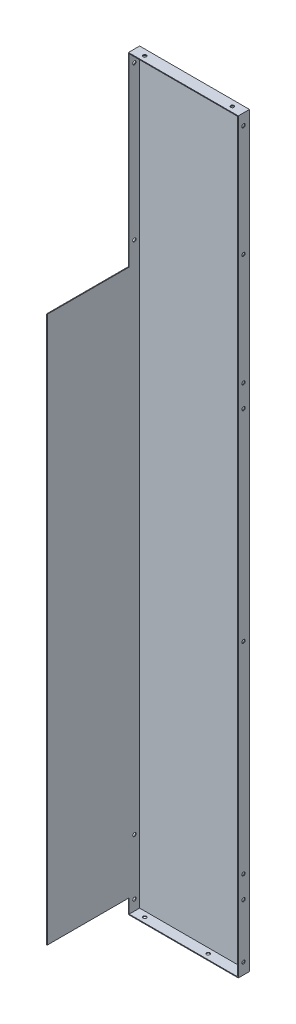
from build123d import *

# Parameters (mm, degrees)
SKETCH_1_W          = 295
SKETCH_1_H          = 2005
EXTRUDE_1_DEPTH     = 30
SHELL_1_T           = -2
SKETCH_2_W          = 2
SKETCH_2_H          = 1467
EXTRUDE_2_DEPTH     = 220
SKETCH_3_R          = 4.5
CUT_EXTRUDE_1_DEPTH = 10
SKETCH_4_R          = 4.5
CUT_EXTRUDE_2_DEPTH = 116
SKETCH_5_R          = 4.5
CUT_EXTRUDE_3_DEPTH = 72
SKETCH_6_R          = 4.5
CUT_EXTRUDE_4_DEPTH = 10
CUT_EXTRUDE_START   = -10
SKETCH_7_R          = 4.5
CUT_EXTRUDE_5_DEPTH = 10
SKETCH_8_R          = 4.5
CUT_EXTRUDE_6_DEPTH = 16


with BuildPart() as part:
    # 草图1 → 凸台-拉伸1 (new body)
    with BuildSketch(Plane.XY):
        with Locations((147.5, 1002.5)):
            Rectangle(SKETCH_1_W, SKETCH_1_H)
    extrude(amount=EXTRUDE_1_DEPTH)

    # 抽壳1
    shell_1_openings = [part.faces().sort_by_distance(p)[0] for p in [
        (147.5, 1002.5, 30),
    ]]
    offset(amount=SHELL_1_T, openings=shell_1_openings, kind=Kind.INTERSECTION)

    # 草图2 → 凸台-拉伸2 (add)
    with BuildSketch(Plane.XY.offset(30)):
        with Locations((1, 773.5)):
            Rectangle(SKETCH_2_W, SKETCH_2_H)
    extrude(amount=EXTRUDE_2_DEPTH)

    # 草图3 → 切除-拉伸1 (cut)
    with BuildSketch(Plane(origin=(0, 2, 0), x_dir=(1, 0, 0), z_dir=(0, 1, 0))):
        with Locations(Location((30, -16, 0), (0, 0, 270))):
            Circle(SKETCH_3_R)
        with Locations(Location((200, -16, 0), (0, 0, 270))):
            Circle(SKETCH_3_R)
    extrude(amount=-CUT_EXTRUDE_1_DEPTH, mode=Mode.SUBTRACT)

    # 草图4 → 切除-拉伸2 (cut)
    with BuildSketch(Plane(origin=(2, 0, 0), x_dir=(0, 0, -1), z_dir=(1, 0, 0))):
        with Locations((-16, 30)):
            Circle(SKETCH_4_R)
        with Locations((-16, 180)):
            Circle(SKETCH_4_R)
    extrude(amount=-CUT_EXTRUDE_2_DEPTH, mode=Mode.SUBTRACT)

    # 草图5 → 切除-拉伸3 (cut)
    with BuildSketch(Plane(origin=(2, 0, 0), x_dir=(0, 0, -1), z_dir=(1, 0, 0))):
        with Locations((-16, 1975)):
            Circle(SKETCH_5_R)
        with Locations((-16, 1563)):
            Circle(SKETCH_5_R)
    extrude(amount=-CUT_EXTRUDE_3_DEPTH, mode=Mode.SUBTRACT)

    # 草图6 → 切除-拉伸4 (cut)
    with BuildSketch(Plane(origin=(0, 2005, 0), x_dir=(1, 0, 0), z_dir=(0, 1, 0))):
        with Locations(Location((30, -16, 0), (0, 0, 270))):
            Circle(SKETCH_6_R)
        with Locations(Location((265, -16, 0), (0, 0, 270))):
            Circle(SKETCH_6_R)
    extrude(amount=-CUT_EXTRUDE_4_DEPTH, mode=Mode.SUBTRACT)

    # 草图7 → 切除-拉伸5 (cut)
    with BuildSketch(Plane.ZY.offset(-293).offset(CUT_EXTRUDE_START)):
        with Locations(Location((16, 1975, 0), (0, 0, 180))):
            Circle(SKETCH_7_R)
        with Locations((16, 1676)):
            Circle(SKETCH_7_R)
        with Locations((16, 1377)):
            Circle(SKETCH_7_R)
        with Locations((16, 1317)):
            Circle(SKETCH_7_R)
        with Locations((16, 776)):
            Circle(SKETCH_7_R)
        with Locations((16, 235)):
            Circle(SKETCH_7_R)
    extrude(amount=CUT_EXTRUDE_5_DEPTH, mode=Mode.SUBTRACT)

    # 草图8 → 切除-拉伸6 (cut)
    with BuildSketch(Plane(origin=(295, 0, 0), x_dir=(0, 0, -1), z_dir=(1, 0, 0))):
        with Locations((-16, 30)):
            Circle(SKETCH_8_R)
        with Locations((-16, 175)):
            Circle(SKETCH_8_R)
    extrude(amount=-CUT_EXTRUDE_6_DEPTH, mode=Mode.SUBTRACT)


solid = part.part
